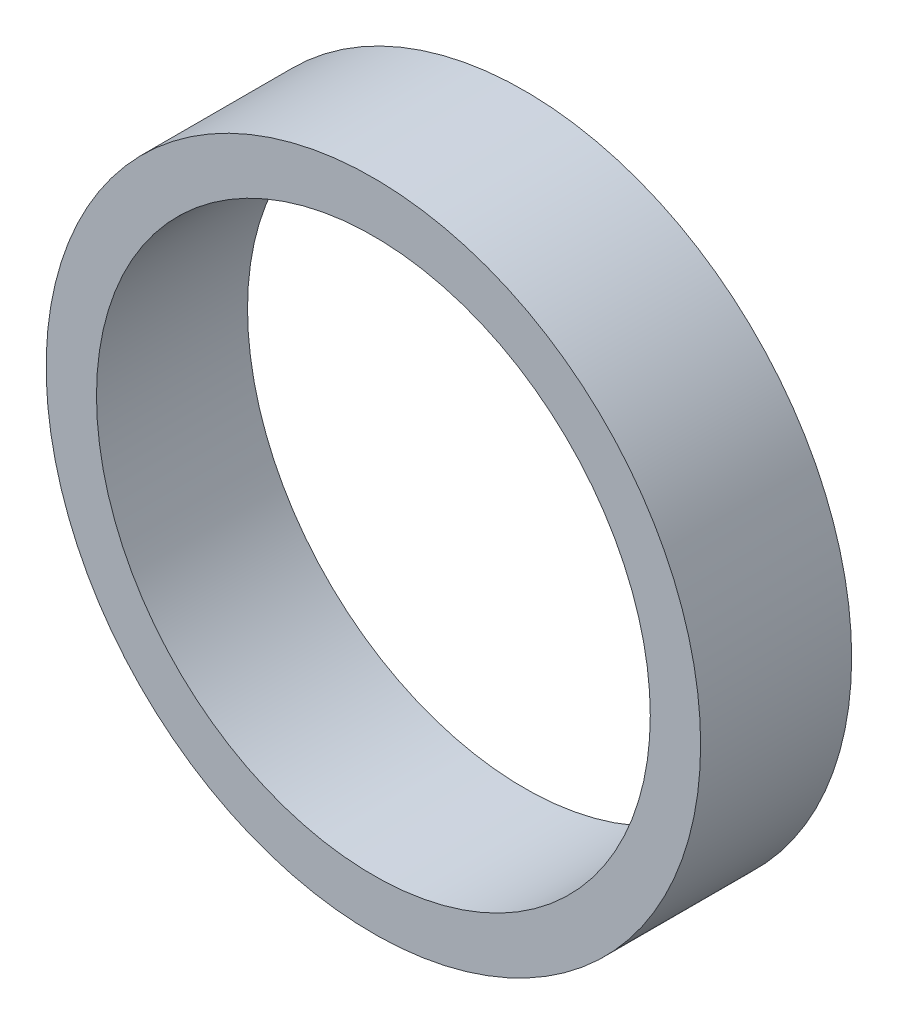
from build123d import *

# Parameters (mm, degrees)
SKETCH1_R           = 13
SKETCH1_R_2         = 11
BOSS_EXTRUDE1_DEPTH = 6


with BuildPart() as part:
    # Sketch1 → Boss-Extrude1 (new body)
    with BuildSketch(Plane.XY):
        Circle(SKETCH1_R)
        Circle(SKETCH1_R_2, mode=Mode.SUBTRACT)
    extrude(amount=BOSS_EXTRUDE1_DEPTH)


solid = part.part
